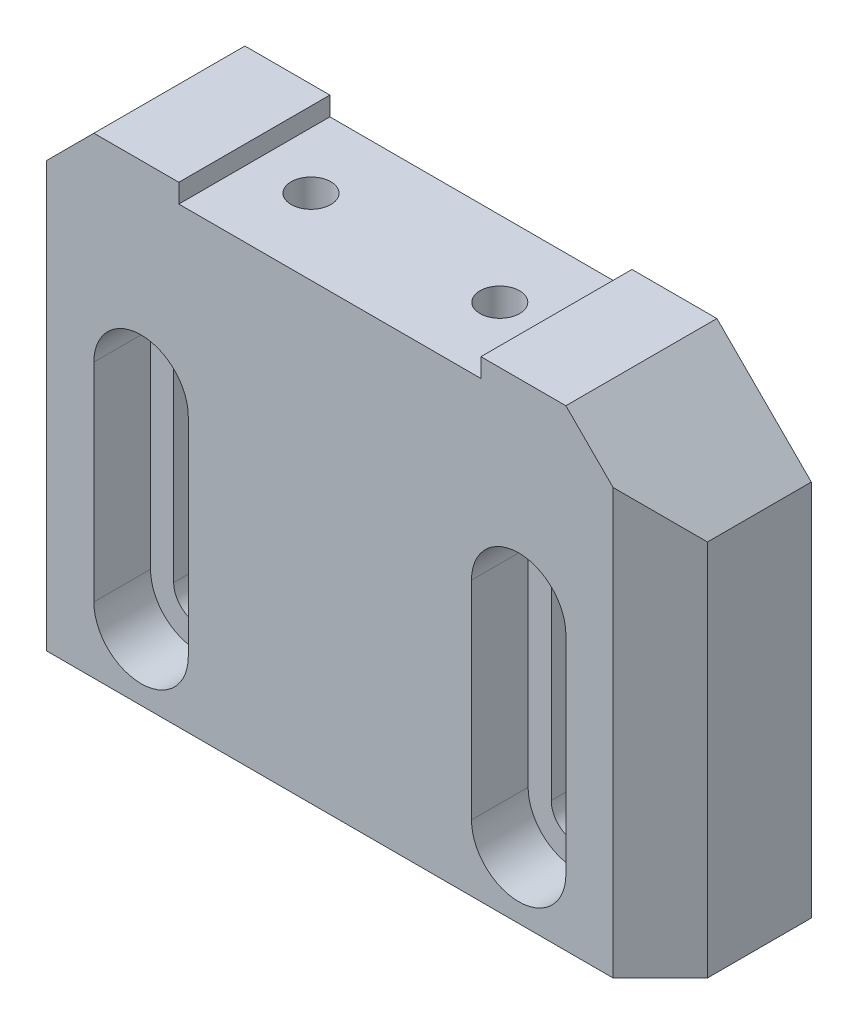
from build123d import *

# Parameters (mm, degrees)
SKETCH1_W             = 70
SKETCH1_H             = 50
EXTRUDE1_DEPTH        = 8
SKETCH2_W             = 32
SKETCH2_H             = 16
EXTRUDE2_DEPTH        = 2
M5_TAPPED_HOLE1_D     = 4.2
M5_TAPPED_HOLE1_DEPTH = 8.4
M5_TAPPED_HOLE1_TIP   = 1.2618073
EXTRUDE3_DEPTH        = 8
EXTRUDE4_DEPTH        = 46.891175622
EXTRUDE5_DEPTH        = 6
CHAMFER1_SIZE         = 10
CHAMFER2_SIZE         = 5


with BuildPart() as part:
    # Sketch1 → Extrude1 (new, symmetric)
    with BuildSketch(Plane.XY):
        Rectangle(SKETCH1_W, SKETCH1_H)
    extrude(amount=EXTRUDE1_DEPTH, both=True)

    # Sketch2 → Extrude2 (cut)
    with BuildSketch(Plane(origin=(0, 25, 0), x_dir=(1, 0, 0), z_dir=(0, 1, 0))):
        Rectangle(SKETCH2_W, SKETCH2_H)
    extrude(amount=-EXTRUDE2_DEPTH, mode=Mode.SUBTRACT)

    # M5 Tapped Hole1
    with Locations(Plane(origin=(0, 23, 0), x_dir=(1, 0, 0), z_dir=(0, 1, 0))):
        with Locations((-10, 0), (10, 0)):
            Hole(M5_TAPPED_HOLE1_D / 2, depth=M5_TAPPED_HOLE1_DEPTH)
            with Locations((0, 0, -(M5_TAPPED_HOLE1_DEPTH + M5_TAPPED_HOLE1_TIP / 2))):  # 118° drill point
                Cone(0, M5_TAPPED_HOLE1_D / 2, M5_TAPPED_HOLE1_TIP, mode=Mode.SUBTRACT)

    # Sketch5 → Extrude3 (cut)
    with BuildSketch(Plane.XY.offset(-8)):
        with BuildLine():
            Line((-33, -25), (33, -25))
            Line((33, -25), (33, 7))
            ThreePointArc((33, 7), (32.121320344, 9.121320344), (30, 10))
            Line((30, 10), (-30, 10))
            ThreePointArc((-30, 10), (-32.121320344, 9.121320344), (-33, 7))
            Line((-33, 7), (-33, -25))
        make_face()
    extrude(amount=EXTRUDE3_DEPTH, mode=Mode.SUBTRACT)

    # Sketch6 → Extrude4 (cut, through all)
    with BuildSketch(Plane.XY.offset(8)):
        with BuildLine():
            Line((-22.55, -18), (-22.55, 4))
            ThreePointArc((-22.55, 4), (-20, 6.55), (-17.45, 4))
            Line((-17.45, 4), (-17.45, -18))
            ThreePointArc((-17.45, -18), (-20, -20.55), (-22.55, -18))
        make_face()
        with BuildLine():
            Line((17.45, -18), (17.45, 4))
            ThreePointArc((17.45, 4), (20, 6.55), (22.55, 4))
            Line((22.55, 4), (22.55, -18))
            ThreePointArc((22.55, -18), (20, -20.55), (17.45, -18))
        make_face()
    extrude(amount=-EXTRUDE4_DEPTH, mode=Mode.SUBTRACT)

    # Sketch7 → Extrude5 (cut)
    with BuildSketch(Plane.XY.offset(8)):
        with BuildLine():
            Line((15, -18), (15, 4))
            ThreePointArc((15, 4), (20, 9), (25, 4))
            Line((25, 4), (25, -18))
            ThreePointArc((25, -18), (20, -23), (15, -18))
        make_face()
        with BuildLine():
            Line((-15, 4), (-15, -18))
            ThreePointArc((-15, -18), (-20, -23), (-25, -18))
            Line((-25, -18), (-25, 4))
            ThreePointArc((-25, 4), (-20, 9), (-15, 4))
        make_face()
    extrude(amount=-EXTRUDE5_DEPTH, mode=Mode.SUBTRACT)

    # Chamfer1
    chamfer1_edges = [part.edges().sort_by_distance(p)[0] for p in [
        (-35, 25, 0),
        (35, 25, 0),
    ]]
    chamfer(chamfer1_edges, length=CHAMFER1_SIZE)

    # Chamfer2
    chamfer2_edges = [part.edges().sort_by_distance(p)[0] for p in [
        (35, -5, 8),
        (-35, -5, 8),
    ]]
    chamfer(chamfer2_edges, length=CHAMFER2_SIZE)


solid = part.part
